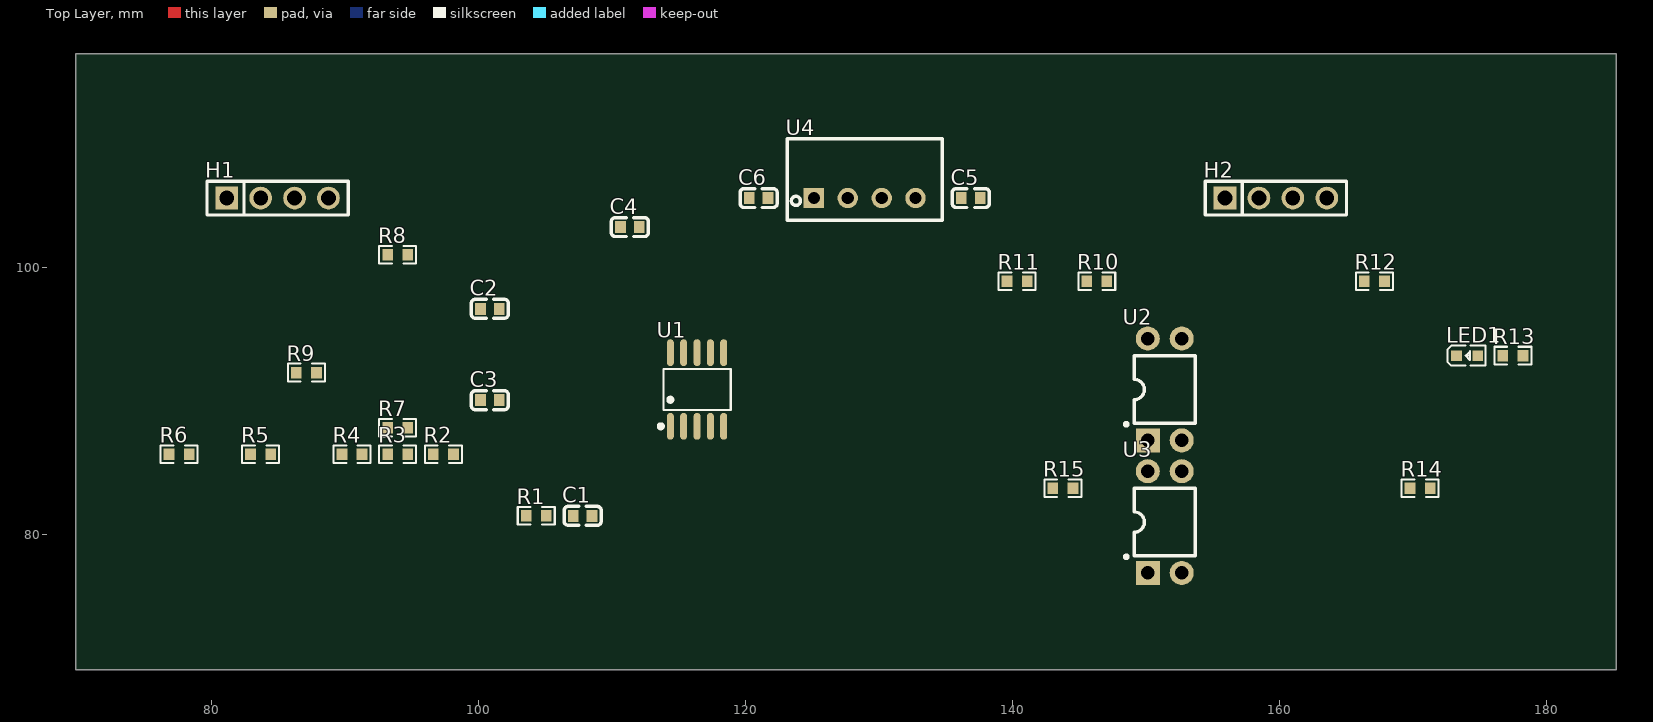
[diagram p0: Top Layer view]
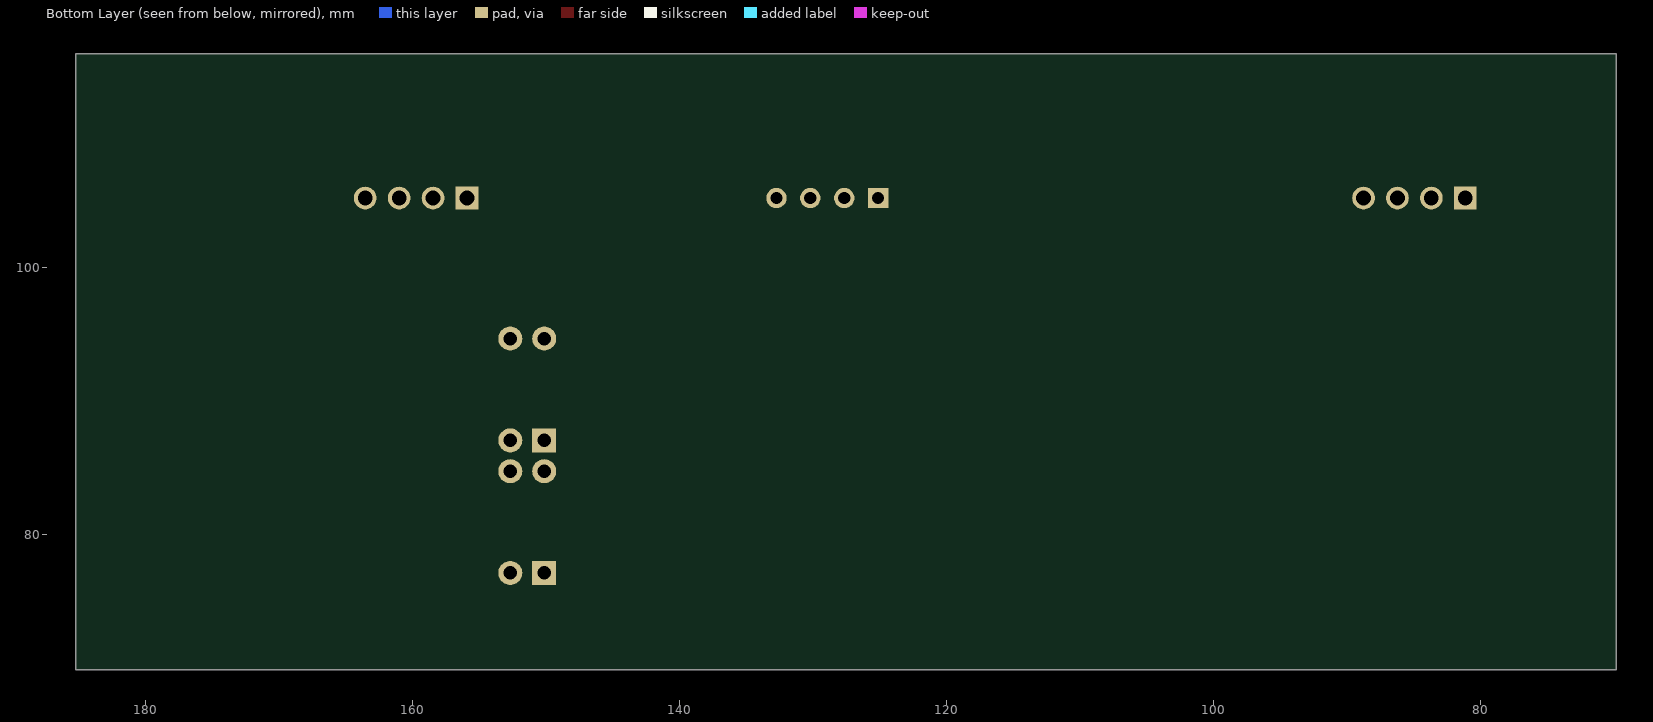
[diagram p1: Bottom Layer view, seen from below]
# Altium PCB MISC51247.pcbdoc
Units mm, origin at the board's own origin, x right, y up, seen from the top; angles counter-clockwise.
Board outline 115.39 x 46.13 mm, 2 copper layers (Top Layer, Bottom Layer), stack 1.58 mm thick; 28 components, 22 nets, 74 pads, 0 vias.

## Layer stack, top to bottom
Top Solder Mask Layer: solder mask 0.01, Dk 3.3
Top Layer: signal copper 0.035
Dielectric1: surface 1.51, FR4, Dk 4.5
Bottom Layer: signal copper 0.035
Bottom Solder Mask Layer: solder mask 0.01, Dk 3.3

## Board outline
185.241,69.85 69.85,69.85 69.85,115.984 185.241,115.984

## Design rules (kind name [scope] priority, off if disabled: settings)
BoardOutlineClearance copperThickness2oz_1 [All] p2 off: genericclearance=0.203 ignorepadtopadclearanceinfootprint=FALSE except(0: Arc-SplitContinuation Track-SplitContinuation SMDPad-SplitContinuation THPad-SplitContinuation Via-SplitContinuation Fill-SplitContinuation Region-SplitContinuation Poly-SplitContinuation Text-SplitContinuation Hole-SplitContinuation; 0.152: Arc-CutoutEdge SMDPad-CutoutEdge THPad-CutoutEdge Via-CutoutEdge Fill-CutoutEdge Region-CutoutEdge Text-CutoutEdge; 0.176: Hole-OutlineEdge Hole-CutoutEdge; 0.254: Poly-OutlineEdge Poly-CutoutEdge; 0.3: Arc-OutlineEdge Track-OutlineEdge SMDPad-OutlineEdge THPad-OutlineEdge Via-OutlineEdge Fill-OutlineEdge Region-OutlineEdge Text-OutlineEdge Track-CutoutEdge)
BoardOutlineClearance copperThickness1oz_1 [All] p4: genericclearance=0.102 ignorepadtopadclearanceinfootprint=FALSE except(0: Arc-SplitContinuation Track-SplitContinuation SMDPad-SplitContinuation THPad-SplitContinuation Via-SplitContinuation Fill-SplitContinuation Region-SplitContinuation Poly-SplitContinuation Text-SplitContinuation Hole-SplitContinuation; 0.152: SMDPad-CutoutEdge THPad-CutoutEdge Via-CutoutEdge Fill-CutoutEdge Region-CutoutEdge Text-CutoutEdge; 0.176: Hole-OutlineEdge Hole-CutoutEdge; 0.254: Poly-OutlineEdge Poly-CutoutEdge; 0.3: Arc-OutlineEdge Track-OutlineEdge SMDPad-OutlineEdge THPad-OutlineEdge Via-OutlineEdge Fill-OutlineEdge Region-OutlineEdge Text-OutlineEdge Arc-CutoutEdge Track-CutoutEdge)
Clearance copperThickness2oz [All] p1 off: gap=0.203 ignorepadtopadclearanceinfootprint=FALSE except(0.152: SMDPad-Track SMDPad-SMDPad THPad-Track SMDPad-THPad THPad-THPad Track-Via SMDPad-Via THPad-Via Via-Via Fill-Track Region-Track Fill-SMDPad Region-SMDPad Fill-THPad Region-THPad Fill-Via Region-Via Fill-Fill Fill-Region Region-Region Arc-Track Arc-SMDPad Arc-THPad Arc-Via Fill-Arc Region-Arc Arc-Arc Text-Track SMDPad-Text Text-THPad Text-Via Fill-Text Region-Text Arc-Text Text-Text; 0.176: Hole-Track Hole-SMDPad Hole-THPad Hole-Via Fill-Hole Region-Hole Hole-Arc Hole-Text; 0.254: Poly-Track Poly-SMDPad Poly-THPad Poly-Via Poly-Fill Poly-Region Poly-Poly Poly-Arc Poly-Text Poly-Hole)
Clearance copperThickness1oz [All] p3: gap=0.102 ignorepadtopadclearanceinfootprint=FALSE except(0.152: SMDPad-Track SMDPad-SMDPad THPad-Track SMDPad-THPad THPad-THPad Track-Via SMDPad-Via THPad-Via Via-Via Fill-Track Region-Track Fill-SMDPad Region-SMDPad Fill-THPad Region-THPad Fill-Via Region-Via Fill-Fill Fill-Region Region-Region Arc-Track Arc-SMDPad Arc-THPad Arc-Via Fill-Arc Region-Arc Arc-Arc Text-Track SMDPad-Text Text-THPad Text-Via Fill-Text Region-Text Arc-Text Text-Text; 0.176: Hole-Track Hole-SMDPad Hole-THPad Hole-Via Fill-Hole Region-Hole Hole-Arc Hole-Text; 0.254: Poly-Track Poly-SMDPad Poly-THPad Poly-Via Poly-Fill Poly-Region Poly-Poly Poly-Arc Poly-Text Poly-Hole)
Creepage creepage [All] p1: checkdistance=0 ignoreinternallayers=TRUE applytopolygonpour=TRUE
DiffPairsRouting differentialPair [All] p1: maxlimit=0.152 minlimit=0.152 mostfreqgap=0.152 toplayer_minwidth=0.127 toplayer_prefwidth=0.254 toplayer_maxwidth=2.54 toplayer_mingap=0.152 toplayer_prefgap=0.152 toplayer_maxgap=0.152 bottomlayer_minwidth=0.127 bottomlayer_prefwidth=0.254 bottomlayer_maxwidth=2.54 bottomlayer_mingap=0.152 bottomlayer_prefgap=0.152 bottomlayer_maxgap=0.152 maxuncoupledlength=0.254
HoleToHoleClearance otherClearance [All] p1: gap=0.3 allowstackedmicrovias=TRUE
Length netLength [All] p1: minlimit=0 maxlimit=0
MatchedLengths netLengthTolerance [All] p1: tolerance=25.4
PasteMaskExpansion pasteMaskExpansion [All] p1: expansion=0
PlaneConnect innerPlane [All] p1: planeconnectstyle=Relief reliefexpansion=0.508 reliefentries=4 reliefconductorwidth=0.254 reliefairgap=0.254
PolygonConnect copperRegion [All] p1: connectstyle=Relief reliefconductorwidth=0.254 reliefentries=4 polygonreliefangle="90 Angle" airgapwidth=0.254 via.connectstyle=Relief via.reliefconductorwidth=0.254 via.reliefentries=4 via.polygonreliefangle="90 Angle" via.airgapwidth=0.254
RoutingVias viaSize [All] p1: holewidth=0.305 width=0.61 viastyle="Through Hole" minholewidth=0.3 minwidth=0.5 maxholewidth=6.3 maxwidth=10
SolderMaskExpansion solderMaskExpansion [IsVia] p1: expansion=-25.4 istentingtop=TRUE
SolderMaskExpansion solderMaskExpansion [All] p2: expansion=0.051 istentingtop=FALSE
Width copperThickness2oz_2 [All] p1 off: maxlimit=2.54 minlimit=0.203 preferedwidth=0.254
Width copperThickness1oz_2 [All] p2: maxlimit=2.54 minlimit=0.127 preferedwidth=0.254

## Components (designator, comment, footprint, x,y, rotation, side; value= is the part's Value field where it differs from the comment)
C1 "68nF" C0603 107.818,81.376 r0 top
C2 "68nF" C0603 100.862,96.888 r0 top
C3 "68nF" C0603 100.862,90.037 r0 top
C4 "100nF" C0603 111.352,103.01 r0 top
C5 "100nF" C0603 136.892,105.184 r0 top
C6 "100nF" C0603 121.004,105.184 r0 top
H1 "" HDR-TH_4P-P2.54-V-F 84.963,105.184 r0 top
H2 "" HDR-TH_4P-P2.54-V-F 159.755,105.184 r0 top
LED1 "" LED_0603 174.132,93.381 r0 top
R1 "510R" R0603 104.34,81.376 r0 top
R2 "390K" R0603 97.384,85.99 r0 top
R3 "390K" R0603 93.961,85.99 r0 top
R4 "390K" R0603 90.539,85.99 r0 top
R5 "390K" R0603 83.693,85.99 r0 top
R6 "390K" R0603 77.585,85.99 r0 top
R7 "510R" R0603 93.961,87.964 r0 top
R8 "510R" R0603 93.961,100.936 r0 top
R9 "510R" R0603 87.116,92.111 r0 top
R10 "1K" R0603 146.333,98.962 r0 top
R11 "10K" R0603 140.37,98.962 r0 top
R12 "3.3K" R0603 167.134,98.962 r0 top
R13 "3.3K" R0603 177.506,93.381 r0 top
R14 "10K" R0603 170.556,83.45 r0 top
R15 "1K" R0603 143.793,83.45 r0 top
U1 "BL0942" SSOP-10_L4.9-W3.9-P1.00-LS6.0-BL 116.384,90.841 r0 top
U2 "EL817B" DIP-4_L6.5-W4.6-P2.54-LS7.6-BL 151.425,90.841 r0 top
U3 "EL817B" DIP-4_L6.5-W4.6-P2.54-LS7.6-BL 151.425,80.91 r0 top
U4 "270kHz" PWRM-TH_B0305S-1WR2 128.948,105.184 r0 top

## Footprints (in the part's own frame and the unit in brackets; to place one, negate y for a bottom-side part, rotate by r counter-clockwise, add the part's x,y. Pads: shape width x height; smd on the part's side, far side on the other; paste and mask are expansions set on the pad)
C0603 [mm]
  rect 0.8x0.9 smd: 1(-0.7,0) 2(0.7,0)
  silkscreen extent -1.39,-0.71 1.39,0.71
DIP-4_L6.5-W4.6-P2.54-LS7.6-BL [mm]
  rect 1.8x1.8 hole 1: 1(-1.27,-3.81)
  round 1.8 hole 1: 2(1.27,-3.81) 3(1.27,3.81) 4(-1.27,3.81)
  silkscreen extent -3,-2.73 2.29,2.54
HDR-TH_4P-P2.54-V-F [mm]
  rect 1.7x1.7 hole 1.1: 1(-3.81,0)
  round 1.7 hole 1.1: 2(-1.27,0) 3(1.27,0) 4(3.81,0)
  silkscreen extent -5.29,-1.27 5.29,1.27
LED_0603 [mil]
  rect 31.5x31.5 smd paste+0 mask+2: 1(-33.5,-0.4) 2(29.5,-0.2)
  silkscreen extent -61,-30 53,30
PWRM-TH_B0305S-1WR2 [mil]
  rect 60x60 hole 36: 1(-150,0)
  round 60 hole 36: 2(-50,0) 3(50,0) 4(150,0)
  silkscreen extent -228,-65 228,175
R0603 [mm]
  rect 0.806x0.864 smd paste-100 mask+0.051: 1(-0.753,0) 2(0.753,0)
  silkscreen extent -1.39,-0.66 1.39,0.66
SSOP-10_L4.9-W3.9-P1.00-LS6.0-BL [mm]
  oval 0.525x2.014 smd: 1(-2,-2.757) 2(-1,-2.757) 3(0,-2.757) 4(1,-2.757) 5(2,-2.757) 6(2,2.757) 7(1,2.757) 8(0,2.757) 9(-1,2.757) 10(-2,2.757)
  silkscreen extent -2.86,-2.91 2.53,1.52

## Nets (pads, with @x,y where several pads share a name; then routed paths per layer and width w, separated by ;. In a path a pad name is that pad's centre, name@x,y a point inside that pad or via, vN(x,y) a via of type N, cw(c..) or ccw(c..) an arc to the next point about the centre after c; other vN are vias at no path point)
$1N5: C1.2 R1.2 R2.1 U1.4
$1N9: R2.2 R3.1
$1N10: R3.2 R4.1
$1N11: R4.2 R5.1
$1N12: R5.2 R6.1
$1N15: C3.1 R7.1 U1.3
$1N17: C2.2 R8.1 U1.2
$1N18: R8.2 R9.1
$1N30: R10.2 U2.1
$1N36: LED1.2 R13.1
$1N41: U3.2
$1N42: R15.2 U3.1
GND: C1.1 C2.1 C3.2 C4.1 C6.2 H1.2 R1.1 R7.2 R9.2 U1.5 U3.3 U4.3
IN_3V: C5.2 H2.4 R12.1 R13.2 R15.1 U4.2
INL: H1.1 H1.3 R6.2
OGND: C5.1 H2.1 U2.3 U4.1
ORX: H2.2
OTX: H2.3 LED1.1 R12.2 U2.4
OUT_N: H1.4
RX: R14.1 U1.9 U3.4
TX: R11.2 U1.10 U2.2
VCC: C4.2 C6.1 R10.1 R11.1 R14.2 U1.1 U1.8 U4.4
pads on no net: U1.6 U1.7